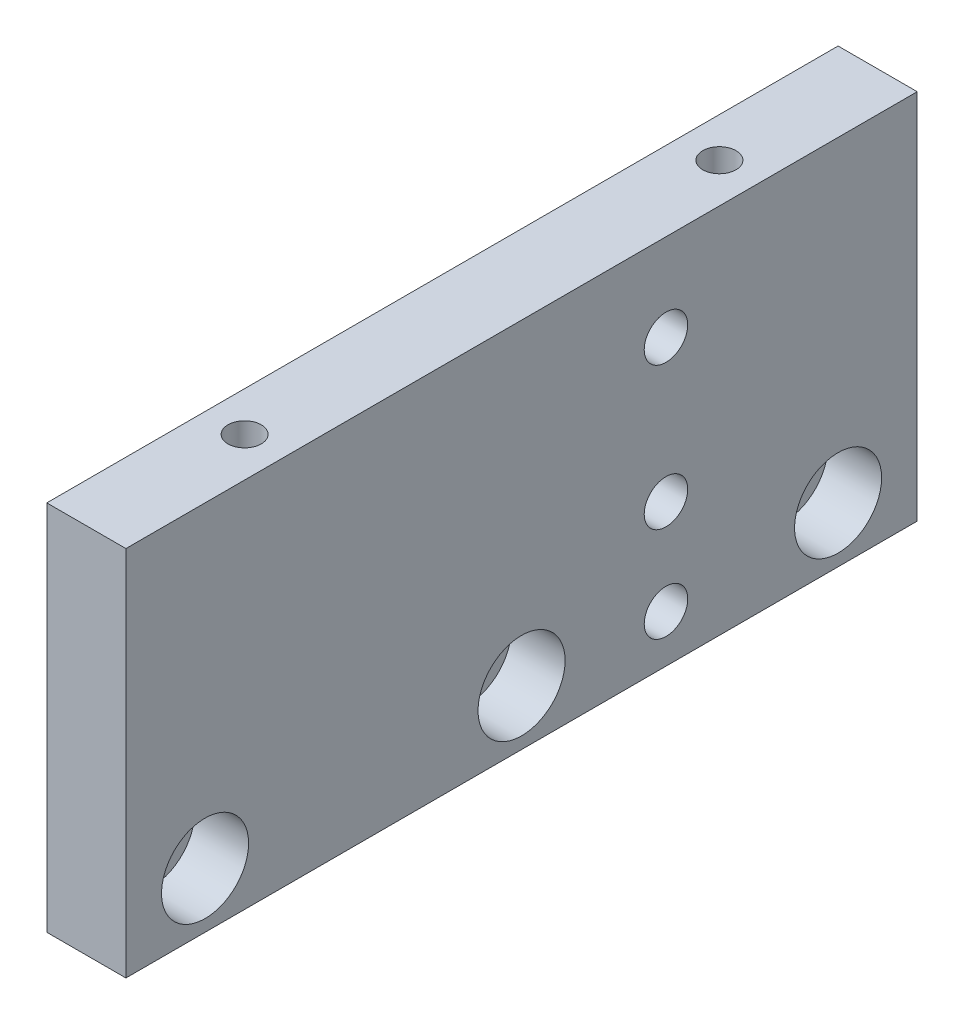
from build123d import *

# Parameters (mm, degrees)
SKETCH_1_W                = 100
SKETCH_1_H                = 47
EXTRUDE_1_DEPTH           = 10
HOLE_WIZARD_1_D           = 6.6
HOLE_WIZARD_1_DEPTH       = 15
HOLE_WIZARD_1_CBORE_D     = 11
HOLE_WIZARD_1_CBORE_DEPTH = 6.8
HOLE_WIZARD_1_TIP         = 1.982840043
HOLE_WIZARD_2_D           = 5.5
HOLE_WIZARD_2_CBORE_D     = 10
HOLE_WIZARD_2_CBORE_DEPTH = 5.7
HOLE_WIZARD_M5_1_D        = 4.2
HOLE_WIZARD_M5_1_DEPTH    = 12.4
HOLE_WIZARD_M5_1_TIP      = 1.2618073


with BuildPart() as part:
    # 草图1 → 凸台-拉伸1 (new body)
    with BuildSketch(Plane(origin=(0, 0, 0), x_dir=(0, 0, -1), z_dir=(1, 0, 0))):
        Rectangle(SKETCH_1_W, SKETCH_1_H)
    extrude(amount=EXTRUDE_1_DEPTH)

    # 打孔尺寸(%根据)内六角圆柱头螺钉的类型1
    with Locations(Plane(origin=(10, 0, 0), x_dir=(0, 0, -1), z_dir=(1, 0, 0))):
        with Locations((-40, -16.5), (0, -16.5), (40, -16.5)):
            CounterBoreHole(HOLE_WIZARD_1_D / 2, HOLE_WIZARD_1_CBORE_D / 2, HOLE_WIZARD_1_CBORE_DEPTH, depth=HOLE_WIZARD_1_DEPTH)
            with Locations((0, 0, -(HOLE_WIZARD_1_DEPTH + HOLE_WIZARD_1_TIP / 2))):  # 118° drill point
                Cone(0, HOLE_WIZARD_1_D / 2, HOLE_WIZARD_1_TIP, mode=Mode.SUBTRACT)

    # 打孔尺寸(%根据)内六角圆柱头螺钉的类型2 (through all)
    with Locations(Plane.ZY):
        with Locations((-18.25, 12.5), (-18.25, -5.5), (-18.25, -17.5)):
            CounterBoreHole(HOLE_WIZARD_2_D / 2, HOLE_WIZARD_2_CBORE_D / 2, HOLE_WIZARD_2_CBORE_DEPTH)

    # M5 螺纹孔1
    with Locations(Plane(origin=(0, 23.5, 0), x_dir=(1, 0, 0), z_dir=(0, 1, 0))):
        with Locations((5, -30), (5, 30)):
            Hole(HOLE_WIZARD_M5_1_D / 2, depth=HOLE_WIZARD_M5_1_DEPTH)
            with Locations((0, 0, -(HOLE_WIZARD_M5_1_DEPTH + HOLE_WIZARD_M5_1_TIP / 2))):  # 118° drill point
                Cone(0, HOLE_WIZARD_M5_1_D / 2, HOLE_WIZARD_M5_1_TIP, mode=Mode.SUBTRACT)


solid = part.part
